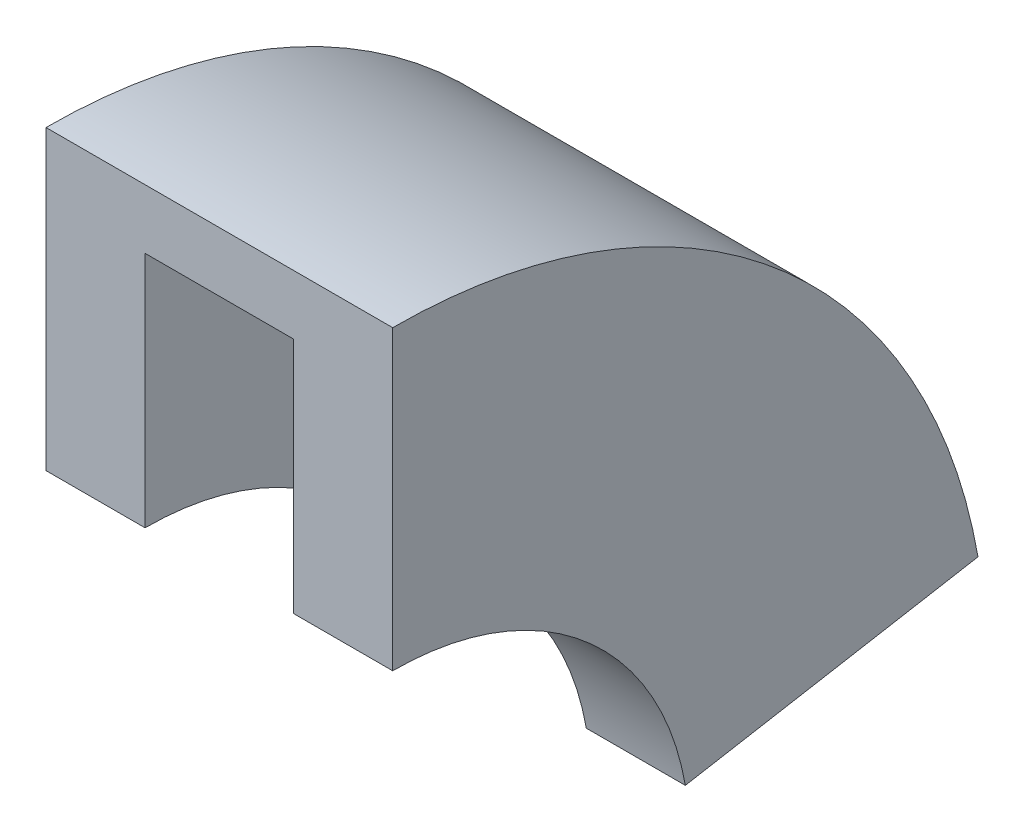
SolidWorks part; units mm, degrees
material "普通碳钢"
ref_plane "Front Plane" through (0, 0, 0) normal (0, 0, 1) x (1, 0, 0)
ref_plane "Top Plane" through (0, 0, 0) normal (0, 1, 0) x (1, 0, 0)
ref_plane "Right Plane" through (0, 0, 0) normal (1, 0, 0) x (0, 0, -1)
sketch "Sketch1" plane through (0, 0, 0) normal (0, 0, 1) x (1, 0, 0)
  line L0 (-0.1364, 58.7166) -> (19.8636, 58.7166)
  line L1 (19.8636, 58.7166) -> (19.8636, 118.7166)
  line L2 (-50.1364, 118.7166) -> (19.8636, 118.7166)
  line L3 (-0.1364, 58.7166) -> (-0.1364, 106.7166)
  line L4 (-0.1364, 106.7166) -> (-30.1364, 106.7166)
  line L5 (-30.1364, 106.7166) -> (-30.1364, 58.7166)
  line L6 (-30.1364, 58.7166) -> (-50.1364, 58.7166)
  line L7 (-50.1364, 58.7166) -> (-50.1364, 118.7166)
  line L8 (-15.1364, 63.8673) -> (-15.1364, 144.6592) construction
  line L9 (39.5415, -1.2834) -> (-147.898, -1.2834) construction
  dimension "D1" = 15
  dimension "D2" = 15
  dimension "D3" = 20
  dimension "D4" = 120
  dimension "D5" = 60
  dimension "D6" = 60
  dimension "D7" = 20
  dimension "D8" = 12
revolve "Revolve1" add sketch "Sketch1" angle 80 about L9
sketch "Sketch3" plane through (-50.1364, 0, 0) normal (-1, 0, 0) x (0, 0, 1)
  line L0 (-38.5673, 44.6792) -> (-77.1345, 90.6419) construction
  arc A0 (0, 58.7166) -> (-59.0885, 9.1354) centre (0, -1.2834) ccw construction
  arc A1 (0, 118.7166) -> (-118.1769, 19.5543) centre (0, -1.2834) ccw construction
  circle A2 centre (-48.2091, 56.1699) radius 7.5
  dimension "D1" = 15
  dimension "D2" = 15
extrude "Boss-Extrude1" add sketch "Sketch3" along normal blind 10
shell "Shell3" thickness 5
sketch "Sketch4" plane through (-30.1364, 0, 0) normal (1, 0, 0) x (0, 0, -1)
  line L0 (38.5673, 44.6792) -> (77.1345, 90.6419) construction
  arc A0 (118.1769, 19.5543) -> (0, 118.7166) centre (0, -1.2834) ccw construction
  arc A1 (59.0885, 9.1354) -> (0, 58.7166) centre (0, -1.2834) ccw construction
  circle A4 centre (52.7086, 61.5322) radius 15
  dimension "D1" = 30
  dimension "D2" = 22
extrude "Cut-Extrude1" cut sketch "Sketch4" against normal up to next and the other way up to next
